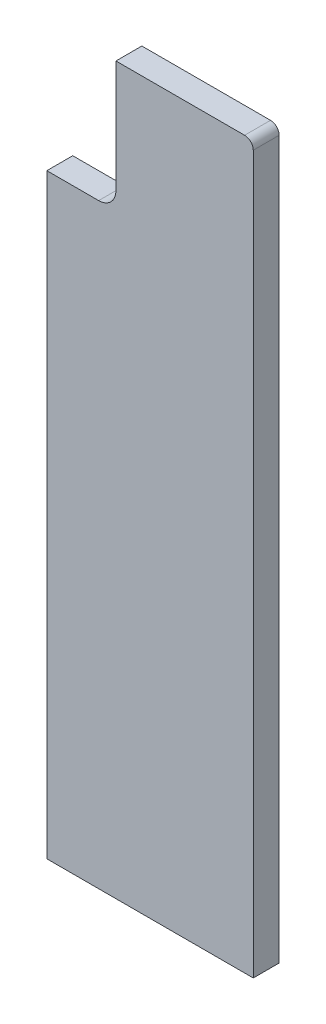
SolidWorks part; units mm, degrees
material "Q235B"
ref_plane "Front Plane" through (0, 0, 0) normal (0, 0, 1) x (1, 0, 0)
ref_plane "Top Plane" through (0, 0, 0) normal (0, 1, 0) x (1, 0, 0)
ref_plane "Right Plane" through (0, 0, 0) normal (1, 0, 0) x (0, 0, -1)
sketch "Sketch1" plane through (0, 0, 0) normal (0, 0, 1) x (1, 0, 0)
  line L0 (0, 0) -> (239, 0)
  line L1 (239, 0) -> (239, 840)
  line L2 (239, 840) -> (80, 840)
  line L3 (0, 690) -> (0, 0)
  line L4 (0, 690) -> (60, 690)
  line L5 (80, 710) -> (80, 840)
  arc A0 (60, 690) -> (80, 710) centre (60, 710) ccw
  point P9 (80, 690)
  dimension "D6" = 20
  dimension "D1" = 239
  dimension "D2" = 840
  dimension "D3" = 239
  dimension "D4" = 80
  dimension "D5" = 150
extrude "Boss-Extrude1" add sketch "Sketch1" along normal blind 30
fillet "Fillet1" radius 10 1 edges at (239, 840, 15)
